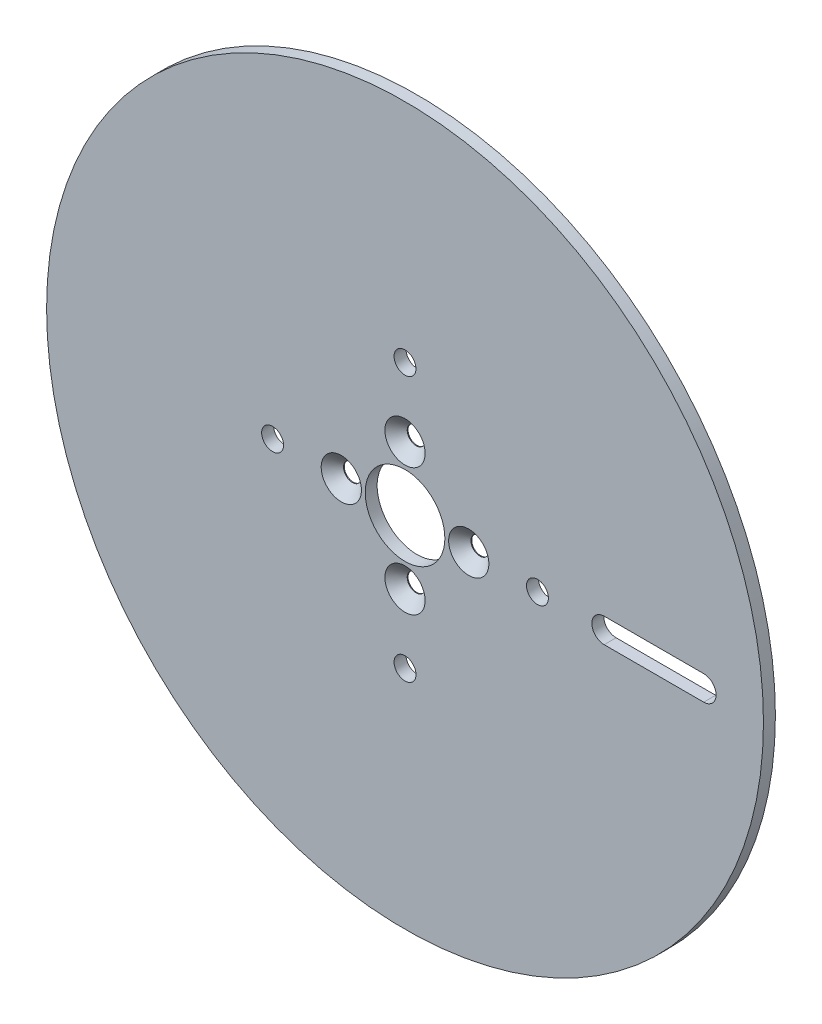
SolidWorks part; units mm, degrees
ref_plane "Front" through (0, 0, 0) normal (0, 0, 1) x (1, 0, 0)
ref_plane "Top" through (0, 0, 0) normal (0, 1, 0) x (1, 0, 0)
ref_plane "Right" through (0, 0, 0) normal (1, 0, 0) x (0, 0, -1)
sketch "Sketch1" plane through (0, 0, 0) normal (0, 0, 1) x (1, 0, 0)
  circle A0 centre (0, 0) radius 90
  circle A1 centre (0, 0) radius 10
  dimension "D1" = 20
  dimension "D2" = 180
extrude "Boss-Extrude1" add sketch "Sketch1" along normal blind 3
sketch "Sketch2" plane through (0, 0, 3) normal (0, 0, 1) x (1, 0, 0)
  line L0 (50, 0) -> (75, 0) construction
  line L1 (50, 3.1) -> (75, 3.1)
  line L2 (50, -3.1) -> (75, -3.1)
  circle A0 centre (0, 0) radius 16 construction
  circle A1 centre (0, 0) radius 33.25 construction
  circle A2 centre (0, 16) radius 2.25
  circle A3 centre (-16, 0) radius 2.25
  circle A4 centre (0, -16) radius 2.25
  circle A5 centre (16, 0) radius 2.25
  circle A6 centre (0, 33.25) radius 2.75
  circle A7 centre (-33.25, 0) radius 2.75
  circle A8 centre (0, -33.25) radius 2.75
  circle A9 centre (33.25, 0) radius 2.75
  arc A10 (50, 3.1) -> (50, -3.1) centre (50, 0) ccw
  arc A11 (75, -3.1) -> (75, 3.1) centre (75, 0) ccw
  circle A12 centre (0, 0) radius 10 construction
  point P22 (62.5, 0)
  dimension "D1" = 32
  dimension "D2" = 66.5
  dimension "D3" = 4.5
  dimension "D4" = 5.5
  dimension "D7" = 50
  dimension "D5" = 6.2
  dimension "D6" = 25
extrude "Cut-Extrude1" cut sketch "Sketch2" against normal blind 3
chamfer "Chamfer1" distance 2.8 angle 45 4 edges at (2.25, -16, 3) (18.25, 0, 3) (2.25, 16, 3) (-13.75, 0, 3)
